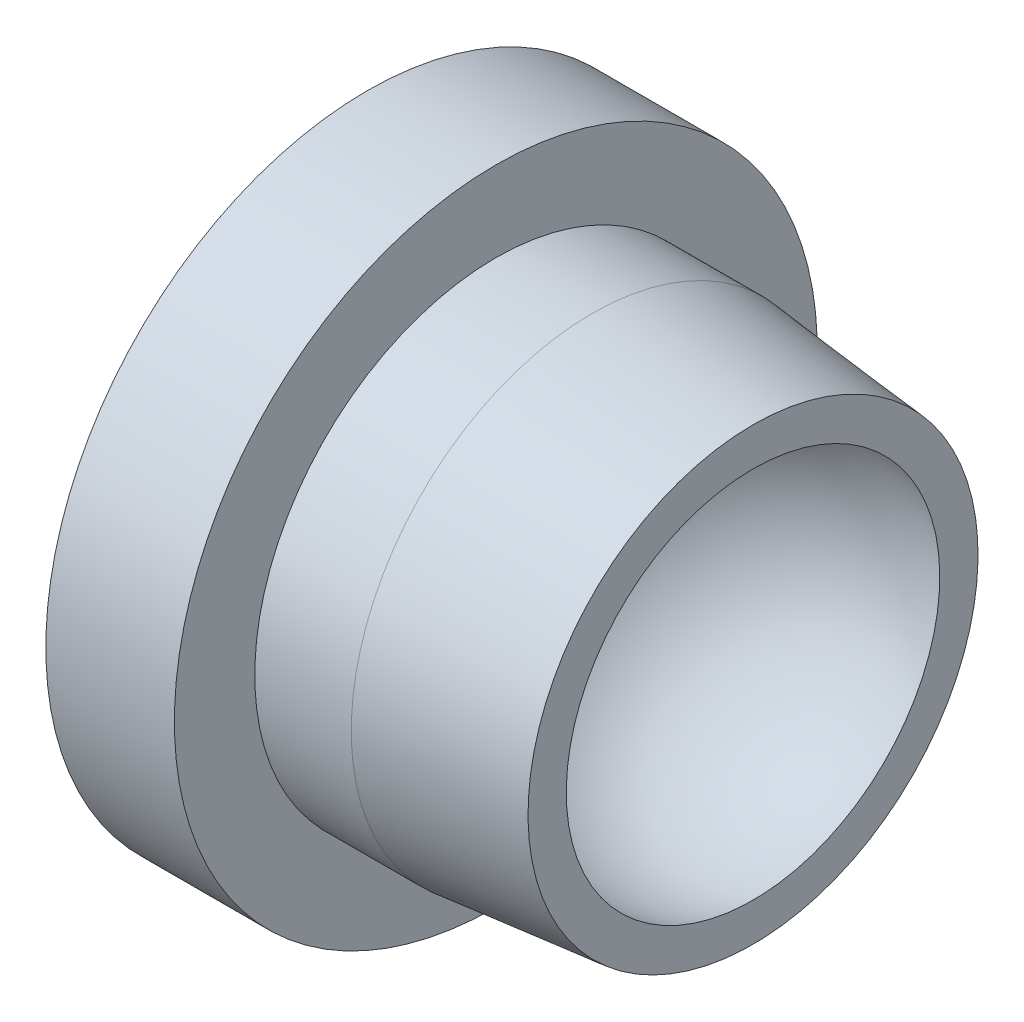
from build123d import *

# Parameters (mm, degrees)
SKETCH2_R          = 4
CUT_EXTRUDE1_DEPTH = 2
SKETCH3_R          = 0.5
CUT_EXTRUDE2_DEPTH = 15
CUT_EXTRUDE3_START = -3.5
SKETCH5_R          = 2
CUT_EXTRUDE3_DEPTH = 15


with BuildPart() as part:
    # Sketch1 → Revolve1 (revolve)
    with BuildSketch(Plane.XY):
        Polygon((0, 0), (0, 10), (4, 10), (4, 7.5), (7, 7.5), (12, 7), (12, 0), align=None)
    revolve(axis=Axis((12, 0, 0), (-1, 0, 0)))

    # Sketch2 → Cut-Extrude1 (cut)
    with BuildSketch(Plane.ZY):
        with Locations(Location((0, 0, 0), (0, 0, 270))):
            Circle(SKETCH2_R)
    extrude(amount=-CUT_EXTRUDE1_DEPTH, mode=Mode.SUBTRACT)

    # Sketch3 → Cut-Extrude2 (cut)
    with BuildSketch(Plane.ZY.offset(-2)):
        with Locations(Location((0, 0, 0), (0, 0, 270))):
            Circle(SKETCH3_R)
    extrude(amount=-CUT_EXTRUDE2_DEPTH, mode=Mode.SUBTRACT)

    # Sketch5 → Cut-Extrude3 (cut)
    with BuildSketch(Plane.ZY.offset(CUT_EXTRUDE3_START)):
        with Locations(Location((0, 0, 0), (0, 0, 270))):
            Circle(SKETCH5_R)
    extrude(amount=-CUT_EXTRUDE3_DEPTH, mode=Mode.SUBTRACT)

    # Sketch6 → Cut-Revolve1 (revolve, cut)
    with BuildSketch(Plane.XY):
        with BuildLine():
            Line((4.5, 0), (16.5, 0))
            ThreePointArc((16.5, 0), (10.5, 6), (4.5, 0))
        make_face()
    revolve(axis=Axis((4.5, 0, 0), (1, 0, 0)), mode=Mode.SUBTRACT)


solid = part.part
